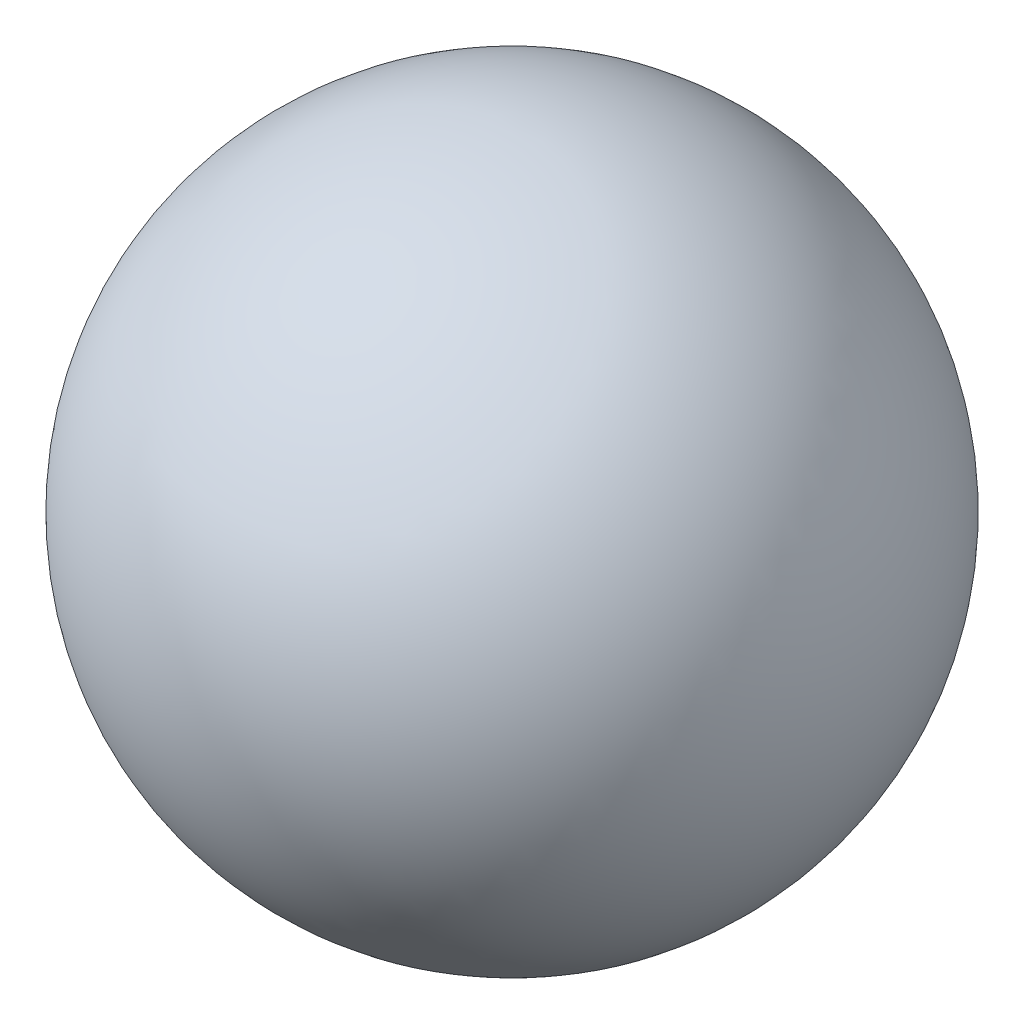
from build123d import *


with BuildPart() as part:
    # 草图1 → 旋转1 (revolve)
    with BuildSketch(Plane.XY):
        with BuildLine():
            Line((0, -8), (0, 8))
            ThreePointArc((0, 8), (-8, 0), (0, -8))
        make_face()
    revolve(axis=Axis((0, 8, 0), (0, -1, 0)))


solid = part.part
